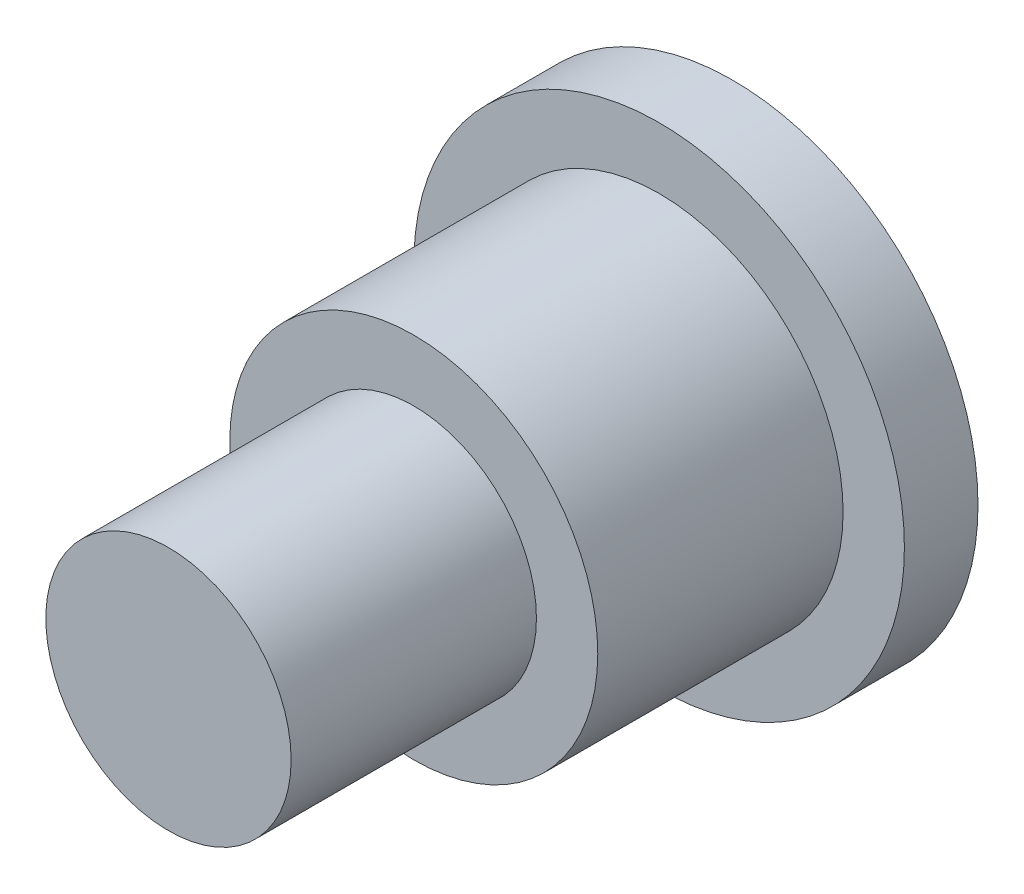
SolidWorks part; units mm, degrees
material "20#"
ref_plane "Front Plane" through (0, 0, 0) normal (0, 0, 1) x (1, 0, 0)
ref_plane "Top Plane" through (0, 0, 0) normal (0, 1, 0) x (1, 0, 0)
ref_plane "Right Plane" through (0, 0, 0) normal (1, 0, 0) x (0, 0, -1)
sketch "Sketch1" plane through (0, 0, 0) normal (1, 0, 0) x (0, 0, -1)
  line L0 (0, 0) -> (23, 0) construction
  line L1 (23, 0) -> (23, 10)
  line L2 (23, 10) -> (20, 10)
  line L3 (20, 10) -> (20, 7.5)
  line L4 (10, 5) -> (0, 5)
  line L5 (0, 5) -> (0, 0)
  line L6 (10, 5) -> (10, 7.5)
  line L7 (10, 7.5) -> (20, 7.5)
  line L8 (0, 0) -> (23, 0)
  dimension "D1" = 3
  dimension "D2" = 10
  dimension "D3" = 20
  dimension "D4" = 10
  dimension "D5" = 10
  dimension "D6" = 15
revolve "Revolve1" add sketch "Sketch1" angle 360 about L0
cosmetic thread "Cosmetic Thread1" parameters "D1"=10, "D2"=8.376
